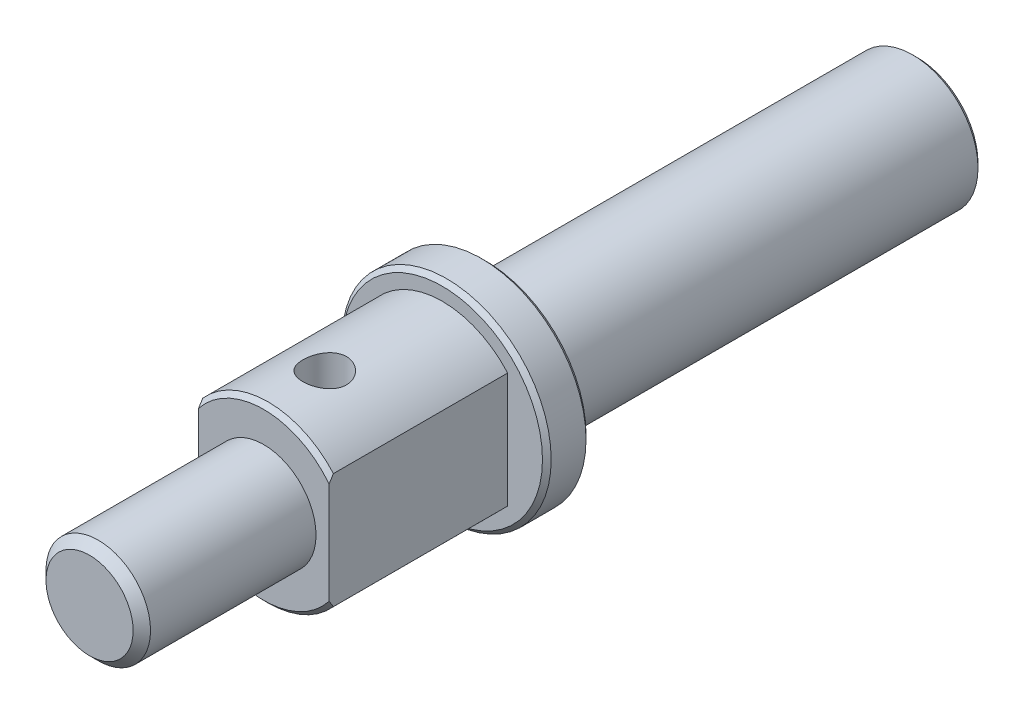
from build123d import *

# Parameters (mm, degrees)
SKETCH_1_R             = 7.5
EXTRUDE_1_DEPTH        = 49.5
SKETCH_2_R             = 12
EXTRUDE_2_DEPTH        = 5
SKETCH_3_R             = 10
EXTRUDE_3_DEPTH        = 20.5
SKETCH_4_R             = 6
EXTRUDE_4_DEPTH        = 20
HOLE_WIZARD_M6_1_D     = 5
HOLE_WIZARD_M6_1_DEPTH = 15
HOLE_WIZARD_M6_1_TIP   = 1.502151548
CHAMFER_1_SIZE         = 0.5
CHAMFER_2_SIZE         = 1
CHAMFER_3_SIZE         = 0.5
SKETCH_7_W             = 26.460285879
SKETCH_7_H             = 26.47281766
SKETCH_7_W_2           = 19.498728734
SKETCH_7_H_2           = 28.747669346
CUT_EXTRUDE_1_DEPTH    = 52
HOLE_WIZARD_M6_2_D     = 5


with BuildPart() as part:
    # 草图1 → 凸台-拉伸1 (new body)
    with BuildSketch(Plane.XY):
        Circle(SKETCH_1_R)
    extrude(amount=EXTRUDE_1_DEPTH)

    # 草图2 → 凸台-拉伸2 (add)
    with BuildSketch(Plane.XY.offset(49.5)):
        Circle(SKETCH_2_R)
    extrude(amount=EXTRUDE_2_DEPTH)

    # 草图3 → 凸台-拉伸3 (add)
    with BuildSketch(Plane.XY.offset(54.5)):
        Circle(SKETCH_3_R)
    extrude(amount=EXTRUDE_3_DEPTH)

    # 草图4 → 凸台-拉伸4 (add)
    with BuildSketch(Plane.XY.offset(75)):
        Circle(SKETCH_4_R)
    extrude(amount=EXTRUDE_4_DEPTH)

    # M6 螺纹孔1
    with Locations(Plane(origin=(0, 0, 0), x_dir=(-1, 0, 0), z_dir=(0, 0, -1))):
        with Locations((0, 0)):
            Hole(HOLE_WIZARD_M6_1_D / 2, depth=HOLE_WIZARD_M6_1_DEPTH)
            with Locations((0, 0, -(HOLE_WIZARD_M6_1_DEPTH + HOLE_WIZARD_M6_1_TIP / 2))):  # 118° drill point
                Cone(0, HOLE_WIZARD_M6_1_D / 2, HOLE_WIZARD_M6_1_TIP, mode=Mode.SUBTRACT)

    # 倒角1
    chamfer_1_edges = [part.edges().sort_by_distance(p)[0] for p in [
        (-7.5, 0, 0),
        (-12, 0, 49.5),
        (-12, 0, 54.5),
    ]]
    chamfer(chamfer_1_edges, length=CHAMFER_1_SIZE)

    # 倒角2
    chamfer_2_edges = [part.edges().sort_by_distance(p)[0] for p in [
        (-6, 0, 95),
    ]]
    chamfer(chamfer_2_edges, length=CHAMFER_2_SIZE)

    # 倒角3
    chamfer_3_edges = [part.edges().sort_by_distance(p)[0] for p in [
        (-10, 0, 75),
    ]]
    chamfer(chamfer_3_edges, length=CHAMFER_3_SIZE)

    # 草图7 → 切除-拉伸1 (cut, symmetric)
    with BuildSketch(Plane(origin=(0, 0, 0), x_dir=(1, 0, 0), z_dir=(0, 1, 0))):
        with Locations((-20.73014294, -67.73640883)):
            Rectangle(SKETCH_7_W, SKETCH_7_H)
        with Locations((17.249364367, -68.873834673)):
            Rectangle(SKETCH_7_W_2, SKETCH_7_H_2)
    extrude(amount=CUT_EXTRUDE_1_DEPTH, both=True, mode=Mode.SUBTRACT)

    # M6 螺纹孔2 (through all)
    with Locations(Plane(origin=(0, 10, 0), x_dir=(1, 0, 0), z_dir=(0, 1, 0))):
        with Locations((0, -68)):
            Hole(HOLE_WIZARD_M6_2_D / 2)


solid = part.part
